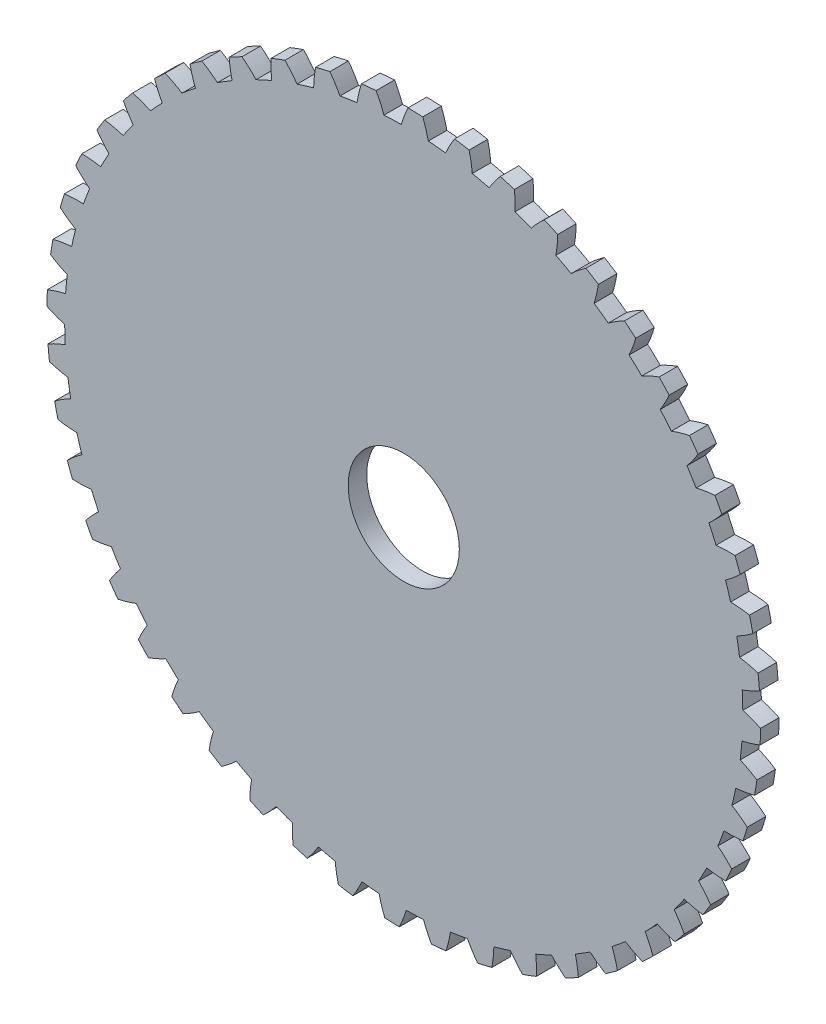
from build123d import *

# Parameters (mm, degrees)
SKETCH1_R           = 9.15
BOSS_EXTRUDE1_DEPTH = 0.5
BOSS_EXTRUDE2_START = -0.5
BOSS_EXTRUDE2_DEPTH = 0.5
CIRPATTERN1_COUNT   = 48
SKETCH3_R           = 1.5
CUT_EXTRUDE1_DEPTH  = 5


with BuildPart() as part:
    # Sketch1 → Boss-Extrude1 (new body)
    with BuildSketch(Plane.XY):
        Circle(SKETCH1_R)
    extrude(amount=BOSS_EXTRUDE1_DEPTH)

    # Sketch2 → Boss-Extrude2 (add)
    with BuildSketch(Plane.XY.offset(0.5).offset(BOSS_EXTRUDE2_START)):
        with BuildLine():
            ThreePointArc((0.513129872, 9.616319344), (0.315084768, 9.624843977), (0.116906155, 9.629290366))
            ThreePointArc((0.116906155, 9.629290366), (0.016073901, 9.393191749), (-0.065494525, 9.149765596))
            ThreePointArc((-0.065494525, 9.149765596), (0.299379608, 9.145100975), (0.663777598, 9.125891699))
            ThreePointArc((0.663777598, 9.125891699), (0.598304648, 9.374131488), (0.513129872, 9.616319344))
        make_face()
    boss_extrude2 = extrude(amount=BOSS_EXTRUDE2_DEPTH)

    # CirPattern1: Boss-Extrude2 ×48 about axis
    cirpattern1_axis = Axis((0, 0, 0), (0, 0, 1))
    for i in range(1, CIRPATTERN1_COUNT):
        add(boss_extrude2.rotate(cirpattern1_axis, i * 360 / CIRPATTERN1_COUNT))

    # Sketch3 → Cut-Extrude1 (cut)
    with BuildSketch(Plane.XY.offset(0.5)):
        Circle(SKETCH3_R)
    extrude(amount=-CUT_EXTRUDE1_DEPTH, mode=Mode.SUBTRACT)


solid = part.part
